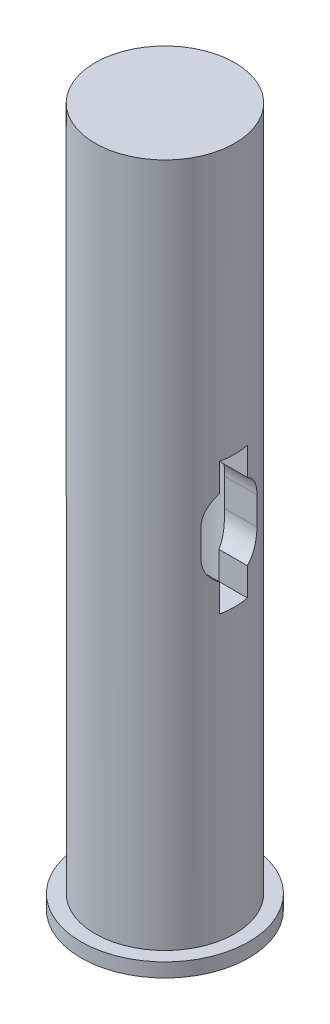
from build123d import *

# Parameters (mm, degrees)
CUT_EXTRUDE1_DEPTH  = 52.23475383
SKETCH9_R           = 6
SKETCH9_R_2         = 3
BOSS_EXTRUDE3_DEPTH = 1
CUT_EXTRUDE2_DEPTH  = 52.546095972


with BuildPart() as part:
    # Sketch3 → Revolve1 (revolve)
    with BuildSketch(Plane.XY, mode=Mode.PRIVATE) as revolve1_sk:
        Polygon((3.025, 0), (3.025, 32.1), (0, 32.1), (0, 50), (5, 50), (5, 0), align=None)
    revolve(revolve1_sk.sketch.rotate(Axis((0, -0.72972973, 0), (0, 1, 0)), 90), axis=Axis((0, -0.72972973, 0), (0, 1, 0)))

    # Sketch6 → Cut-Extrude1 (cut, through all)
    with BuildSketch(Plane(origin=(5, 0, 0), x_dir=(0, 0, -1), z_dir=(1, 0, 0))):
        with BuildLine():
            Line((2, 27), (2, 25))
            ThreePointArc((2, 25), (0, 23), (-2, 25))
            Line((-2, 25), (-2, 27))
            ThreePointArc((-2, 27), (0, 29), (2, 27))
        make_face()
    extrude(amount=-CUT_EXTRUDE1_DEPTH, mode=Mode.SUBTRACT)

    # Sketch9 → Boss-Extrude3 (add)
    with BuildSketch(Plane(origin=(0, 0, 0), x_dir=(1, 0, 0), z_dir=(0, 1, 0))):
        with Locations(Location((0, 0, 0), (0, 0, 270))):
            Circle(SKETCH9_R)
        with Locations(Location((0, 0, 0), (0, 0, 270))):
            Circle(SKETCH9_R_2, mode=Mode.SUBTRACT)
    extrude(amount=BOSS_EXTRUDE3_DEPTH)

    # Sketch11 → Cut-Extrude2 (cut, through all)
    with BuildSketch(Plane(origin=(5, 0, 0), x_dir=(0, 0, -1), z_dir=(1, 0, 0))):
        Polygon((-1, 23.267949192), (-1, 21.267949192), (1, 21.267949192), (1, 23.267949192), (1, 28.732050808), (1, 30.732050808), (-1, 30.732050808), (-1, 28.732050808), align=None)
    extrude(amount=-CUT_EXTRUDE2_DEPTH, mode=Mode.SUBTRACT)


solid = part.part
